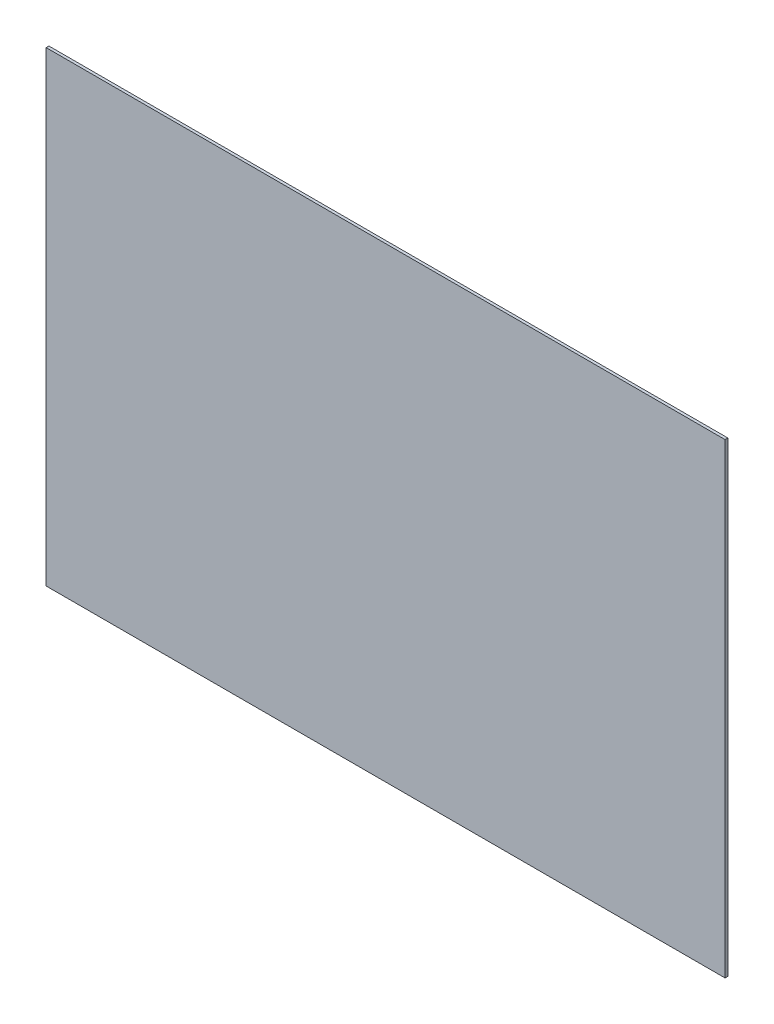
SolidWorks part; units mm, degrees
material "PMMA(有机玻璃)"
ref_plane "前视" through (0, 0, 0) normal (0, 0, 1) x (1, 0, 0)
ref_plane "上视" through (0, 0, 0) normal (0, 1, 0) x (1, 0, 0)
ref_plane "右视" through (0, 0, 0) normal (1, 0, 0) x (0, 0, -1)
sketch "草图1" plane through (0, 0, 0) normal (0, 0, 1) x (1, 0, 0)
  line L1 (-613, 421) -> (613, 421)
  line L2 (-613, 421) -> (-613, -421)
  line L3 (-613, -421) -> (613, -421)
  line L4 (613, 421) -> (613, -421)
  line L5 (-613, 421) -> (613, -421) construction
  line L6 (-613, -421) -> (613, 421) construction
  point P0 (0, 0)
  dimension "D1" = 842
  dimension "D2" = 1226
extrude "凸台-拉伸1" add sketch "草图1" along normal blind 5
hole_wizard "M5 间隙孔1" positions "草图3" profile "草图2" hole size "M5" standard "GB"
sketch "草图3" plane through (0, 0, 5) normal (0, 0, 1) x (1, 0, 0)
  line L0 (-427.5, 273) -> (-427.5, -273) construction
  line L1 (-427.5, -273) -> (427.5, -273) construction
  line L2 (0, 273) -> (0, -273) construction
  line L3 (427.5, 273) -> (-427.5, 273) construction
  line L5 (-427.5, 0) -> (427.5, 0) construction
  line L6 (427.5, -273) -> (427.5, 273) construction
  point P0 (-375, -261)
  point P46 (415.5, 250)
  point P48 (-415.5, 250)
  point P58 (-125, -261)
  point P59 (125, -261)
  point P61 (-125, 261)
  point P62 (125, 261)
  point P64 (-375, 261)
  point P88 (375, -261)
  point P89 (375, 261)
  point P108 (415.5, 0)
  point P109 (-415.5, 0)
  point P110 (415.5, -250)
  point P111 (-415.5, -250)
  dimension "D1" = 12
  dimension "D2" = 12
  dimension "D5" = 3
  dimension "D3" = 12
  dimension "D6" = 4
  dimension "D4" = 2
sketch "草图2" plane through (-375, -261, 5) normal (1, 0, 0) x (0, -1, 0)
  line L0 (0, 0) -> (0, 5)
  line L1 (0, 5) -> (2.75, 5)
  line L2 (2.75, 5) -> (2.75, 0)
  line L5 (2.75, 0) -> (0, 0)
  line L11 (0, -6.35) -> (0, 107.95) construction
  dimension "通孔孔直径" = 5.5
  dimension "通孔孔深度" = 5
